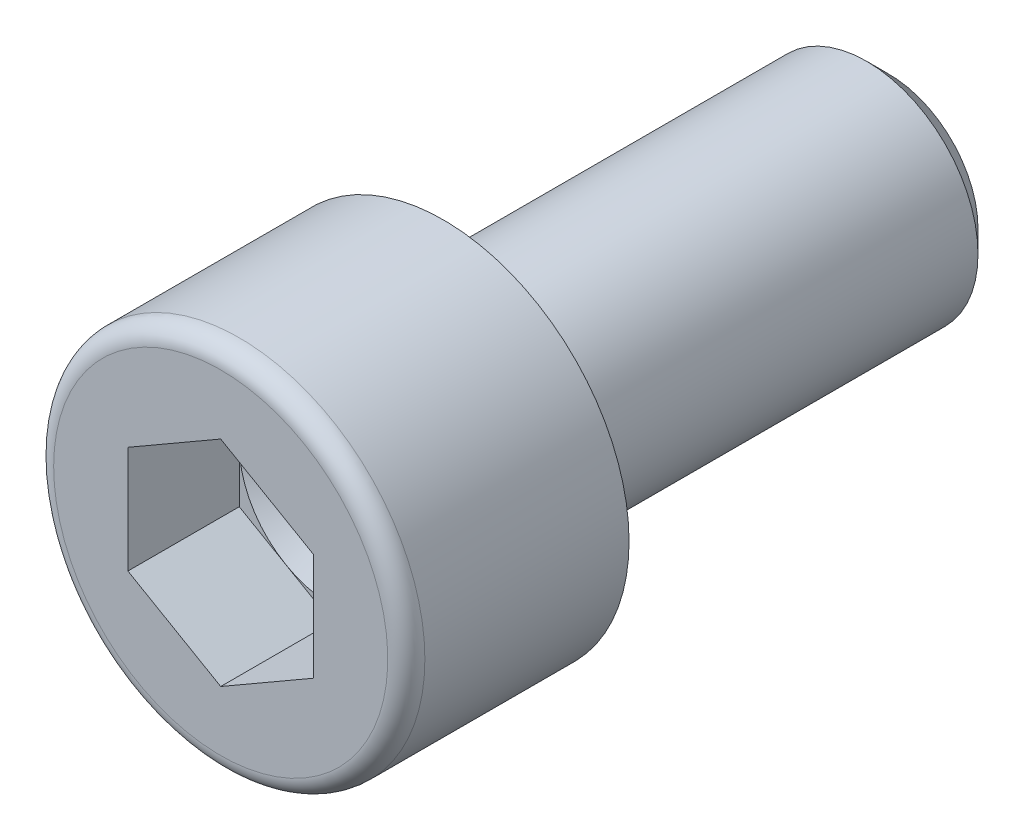
SolidWorks part; units mm, degrees
ref_plane "Front Plane" through (0, 0, 0) normal (0, 0, 1) x (1, 0, 0)
ref_plane "Top Plane" through (0, 0, 0) normal (0, 1, 0) x (1, 0, 0)
ref_plane "Right Plane" through (0, 0, 0) normal (1, 0, 0) x (0, 0, -1)
sketch "Sketch1" plane through (0, 0, 0) normal (1, 0, 0) x (0, 0, -1)
  line L0 (-6, 0) -> (12, 0) construction
  line L1 (-6, 0) -> (-6, 5)
  line L2 (-6, 5) -> (0, 5)
  line L3 (0, 5) -> (0, 3)
  line L4 (0, 3) -> (12, 3)
  line L5 (12, 3) -> (12, 0)
  point P3 (0, 3)
  point P8 (-3, 0)
  point P9 (0.2, 3)
  point P10 (12, 1)
  dimension "A" = 10
  dimension "E" = 6
  dimension "L" = 12
  dimension "M" = 6
  dimension "t" = 3
  dimension "r" = 0.2
  dimension "(d)" = 2
sketch "Sketch2" plane through (0, 0, 0) normal (0, 0, 1) x (1, 0, 0)
  line L1 (0, 2.8868) -> (-2.5, 1.4434)
  line L2 (-2.5, 1.4434) -> (-2.5, -1.4434)
  line L3 (-2.5, -1.4434) -> (0, -2.8868)
  line L4 (0, -2.8868) -> (2.5, -1.4434)
  line L5 (2.5, -1.4434) -> (2.5, 1.4434)
  line L6 (2.5, 1.4434) -> (0, 2.8868)
  circle A0 centre (0, 0) radius 2.5 construction
  dimension "B" = 5
sketch "Sketch3" plane through (0, 0, 0) normal (1, 0, 0) x (0, 0, -1)
  line L0 (-6, 0) -> (-6, 5) construction
  line L1 (-6, 5) -> (0, 5) construction
  line L2 (0, 3) -> (12, 3) construction
  line L3 (0, 5) -> (0, 3) construction
  line L5 (12, 3) -> (12, 0) construction
  line L6 (-6, 1) -> (-6, 5)
  line L7 (-6, 5) -> (0, 5)
  line L8 (0, 3) -> (12, 3)
  line L9 (0, 5) -> (0, 3)
  line L10 (12, 1) -> (-6, 1)
  line L11 (12, 3) -> (12, 1)
revolve "Revolve1" add sketch "Sketch3" angle 360 about L0
cosmetic thread "Cosmetic-Thread1" parameters "D1"=7.8, "D2"=5.1
sketch "Sketch4" plane through (0, 0, 6) normal (0, 0, 1) x (1, 0, 0)
  line L0 (0, 2.8868) -> (-2.5, 1.4434) construction
  line L1 (-2.5, 1.4434) -> (-2.5, -1.4434) construction
  line L2 (-2.5, -1.4434) -> (0, -2.8868) construction
  line L3 (0, -2.8868) -> (2.5, -1.4434) construction
  line L4 (2.5, -1.4434) -> (2.5, 1.4434) construction
  line L5 (2.5, 1.4434) -> (0, 2.8868) construction
  line L6 (0, 2.8868) -> (-2.5, 1.4434)
  line L7 (-2.5, 1.4434) -> (-2.5, -1.4434)
  line L8 (-2.5, -1.4434) -> (0, -2.8868)
  line L9 (0, -2.8868) -> (2.5, -1.4434)
  line L10 (2.5, -1.4434) -> (2.5, 1.4434)
  line L11 (2.5, 1.4434) -> (0, 2.8868)
extrude "Cut-Extrude1" cut sketch "Sketch4" against normal blind 3
fillet "Fillet1" radius 0.5 1 edges at (5, 0, 6)
chamfer "Chamfer1" distance 0.6 angle 45 1 edges at (3, 0, -12)
sketch "Sketch5" plane through (0, 0, 3) normal (0, 0, 1) x (1, 0, 0)
  line L6 (2.5, 1.4434) -> (0, 2.8868)
  line L7 (0, 2.8868) -> (-2.5, 1.4434)
  line L8 (-2.5, 1.4434) -> (-2.5, -1.4434)
  line L9 (-2.5, -1.4434) -> (0, -2.8868)
  line L10 (0, -2.8868) -> (2.5, -1.4434)
  line L11 (2.5, -1.4434) -> (2.5, 1.4434)
  line L12 (2.5, 1.4434) -> (0, 2.8868) construction
  line L13 (0, 2.8868) -> (-2.5, 1.4434) construction
  line L14 (-2.5, 1.4434) -> (-2.5, -1.4434) construction
  line L15 (-2.5, -1.4434) -> (0, -2.8868) construction
  line L16 (0, -2.8868) -> (2.5, -1.4434) construction
  line L17 (2.5, -1.4434) -> (2.5, 1.4434) construction
  circle A0 centre (0, 0) radius 2.5
  dimension "D1" = 0
extrude "Cut-Extrude2" cut sketch "Sketch5" against normal blind 10 draft 60
fillet "Fillet2" radius 0.2 1 edges at (3, 0, 0)
